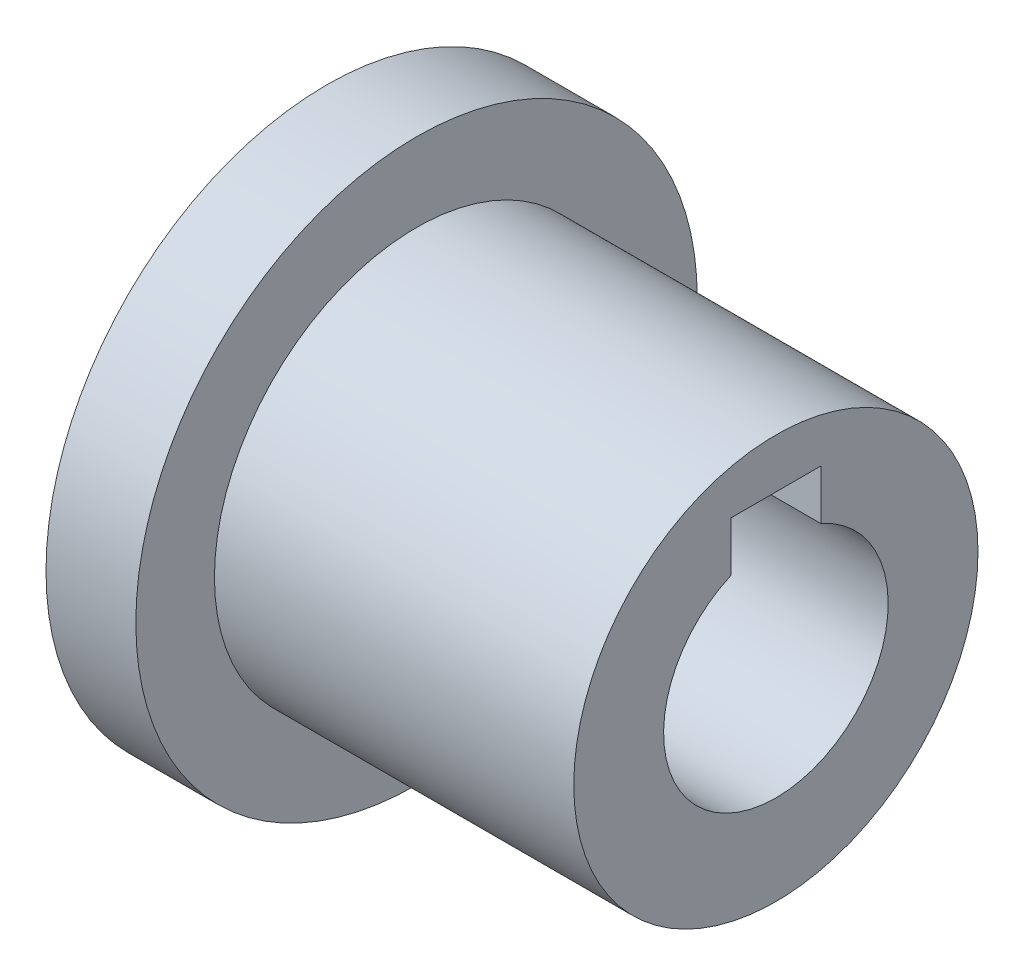
SolidWorks part; units mm, degrees
ref_plane "前视基准面" through (0, 0, 0) normal (0, 0, 1) x (1, 0, 0)
ref_plane "上视基准面" through (0, 0, 0) normal (0, 1, 0) x (1, 0, 0)
ref_plane "右视基准面" through (0, 0, 0) normal (1, 0, 0) x (0, 0, -1)
sketch "草图1" plane through (0, 0, 0) normal (0, 0, 1) x (1, 0, 0)
  line L0 (0, 0) -> (115.0362, 0) construction
  line L1 (0, 5) -> (20, 5)
  line L2 (20, 5) -> (20, 9)
  line L3 (20, 9) -> (4, 9)
  line L4 (4, 9) -> (4, 12.5)
  line L5 (4, 12.5) -> (0, 12.5)
  line L6 (0, 12.5) -> (0, 5)
  dimension "D1" = 5
  dimension "D2" = 20
  dimension "D3" = 4
  dimension "D4" = 4
  dimension "D5" = 3.5
revolve "旋转1" add sketch "草图1" angle 360 about L0
sketch "草图2" plane through (0, 0, 0) normal (-1, 0, 0) x (0, 0, 1)
  line L1 (-2, 0) -> (2, 0)
  line L2 (-2, 0) -> (-2, 6.8)
  line L3 (-2, 6.8) -> (2, 6.8)
  line L4 (2, 0) -> (2, 6.8)
  dimension "D1" = 4
  dimension "D2" = 2
  dimension "D3" = 6.8
extrude "切除-拉伸1" cut sketch "草图2" against normal through all
